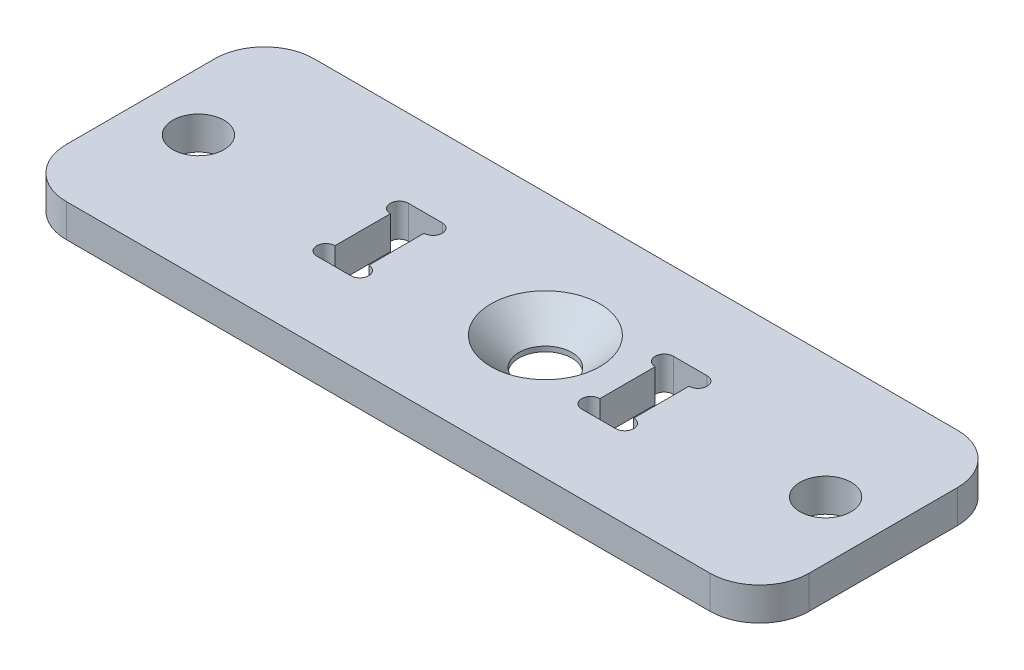
from build123d import *

# Parameters (mm, degrees)
SKETCH_1_W                   = 45
SKETCH_1_H                   = 15
SKETCH_1_R                   = 1.55
EXTRUDE_1_DEPTH              = 2
FILLET_1_R                   = 3
HOLE_WIZARD_M3_1_D           = 3.2
HOLE_WIZARD_M3_1_DEPTH       = 7.5
HOLE_WIZARD_M3_1_CSINK_D     = 6.6
HOLE_WIZARD_M3_1_CSINK_ANGLE = 90
HOLE_WIZARD_M3_1_TIP         = 0.96137699


with BuildPart() as part:
    # 草图1 → 凸台-拉伸1 (new body)
    with BuildSketch(Plane(origin=(0, 0, 0), x_dir=(1, 0, 0), z_dir=(0, 1, 0))):
        Rectangle(SKETCH_1_W, SKETCH_1_H)
        with Locations(Location((-19, 0, 0), (0, 0, 270))):
            Circle(SKETCH_1_R, mode=Mode.SUBTRACT)
        with BuildLine():
            ThreePointArc((-9.05, 1.675), (-9.6, 2.225), (-9.05, 2.775))
            Line((-9.05, 2.775), (-7, 2.775))
            ThreePointArc((-7, 2.775), (-6.61109127, 2.61390873), (-6.45, 2.225))
            ThreePointArc((-6.45, 2.225), (-6.61109127, 1.83609127), (-7, 1.675))
            Line((-7, 1.675), (-7, -1.675))
            ThreePointArc((-7, -1.675), (-6.61109127, -1.83609127), (-6.45, -2.225))
            ThreePointArc((-6.45, -2.225), (-6.61109127, -2.61390873), (-7, -2.775))
            Line((-7, -2.775), (-9.05, -2.775))
            ThreePointArc((-9.05, -2.775), (-9.6, -2.225), (-9.05, -1.675))
            Line((-9.05, -1.675), (-9.05, 1.675))
        make_face(mode=Mode.SUBTRACT)
        with Locations(Location((2.025, 0, 0), (0, 0, 270))):
            Circle(SKETCH_1_R, mode=Mode.SUBTRACT)
        with BuildLine():
            ThreePointArc((7, 1.675), (6.45, 2.225), (7, 2.775))
            Line((7, 2.775), (9.05, 2.775))
            ThreePointArc((9.05, 2.775), (9.43890873, 2.61390873), (9.6, 2.225))
            ThreePointArc((9.6, 2.225), (9.43890873, 1.83609127), (9.05, 1.675))
            Line((9.05, 1.675), (9.05, -1.675))
            ThreePointArc((9.05, -1.675), (9.43890873, -1.83609127), (9.6, -2.225))
            ThreePointArc((9.6, -2.225), (9.43890873, -2.61390873), (9.05, -2.775))
            Line((9.05, -2.775), (7, -2.775))
            ThreePointArc((7, -2.775), (6.45, -2.225), (7, -1.675))
            Line((7, -1.675), (7, 1.675))
        make_face(mode=Mode.SUBTRACT)
        with Locations(Location((19, 0, 0), (0, 0, 270))):
            Circle(SKETCH_1_R, mode=Mode.SUBTRACT)
    extrude(amount=EXTRUDE_1_DEPTH)

    # 圆角1
    fillet_1_edges = [part.edges().sort_by_distance(p)[0] for p in [
        (22.5, 1, 7.5),
        (-22.5, 1, 7.5),
        (-22.5, 1, -7.5),
        (22.5, 1, -7.5),
    ]]
    fillet(fillet_1_edges, radius=FILLET_1_R)

    # M3 十字槽半沉头木螺钉的锥形沉头孔1
    with Locations(Plane(origin=(0, 2, 0), x_dir=(1, 0, 0), z_dir=(0, 1, 0))):
        with Locations((2.025, 0)):
            CounterSinkHole(HOLE_WIZARD_M3_1_D / 2, HOLE_WIZARD_M3_1_CSINK_D / 2, depth=HOLE_WIZARD_M3_1_DEPTH, counter_sink_angle=HOLE_WIZARD_M3_1_CSINK_ANGLE)
            with Locations((0, 0, -(HOLE_WIZARD_M3_1_DEPTH + HOLE_WIZARD_M3_1_TIP / 2))):  # 118° drill point
                Cone(0, HOLE_WIZARD_M3_1_D / 2, HOLE_WIZARD_M3_1_TIP, mode=Mode.SUBTRACT)


solid = part.part
